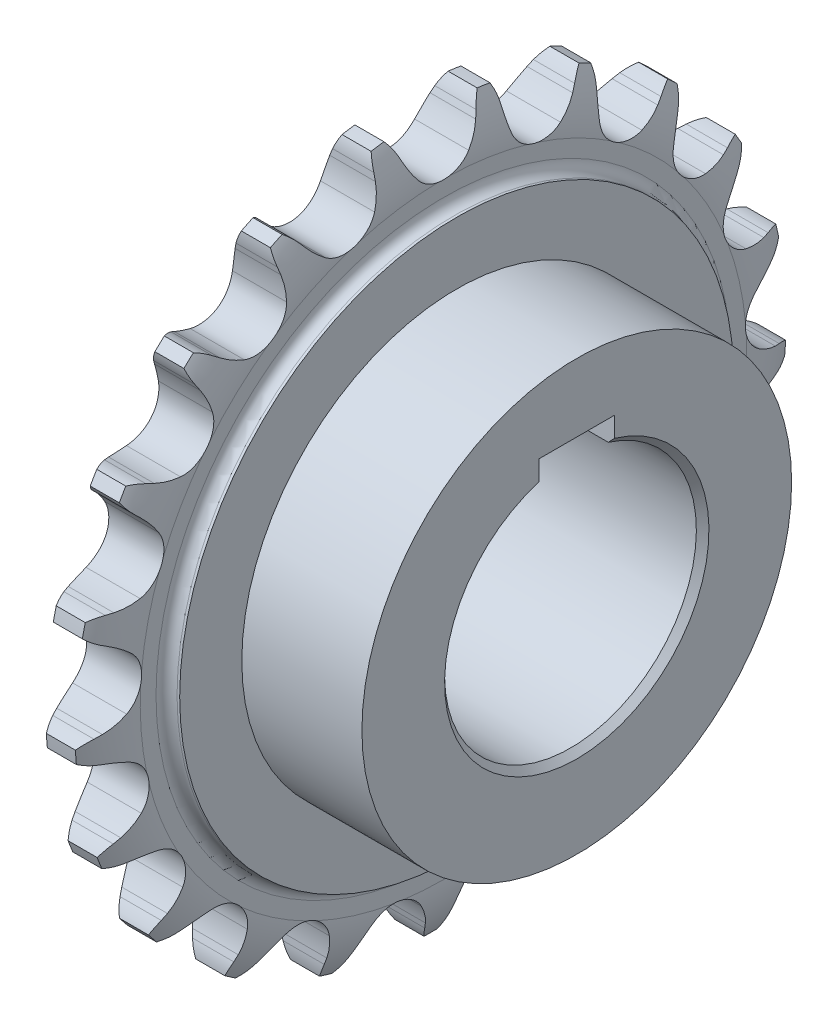
from build123d import *

# Parameters (mm, degrees)
CUT_EXTRUDE_1_DEPTH      = 6.459352492
PATTERN_CIRCULAR_1_COUNT = 21
SKETCH_3_W               = 19.081295016
SKETCH_3_H               = 14.131800766
SKETCH_4_W               = 12
SKETCH_4_H               = 4.221215924
CUT_EXTRUDE_2_DEPTH      = 87.013388292
CHAMFER_1_SIZE           = 1
CHAMFER_3_SIZE           = 1


with BuildPart() as part:
    # 草图1 → 旋转1 (revolve)
    with BuildSketch(Plane.XY, mode=Mode.PRIVATE) as revolve_1_sk:
        with BuildLine():
            Line((-6.459352492, 20), (-6.459352492, 44))
            Line((-6.459352492, 44), (-6.041681994, 44))
            ThreePointArc((-6.041681994, 44), (-4.860331427, 44.489331427), (-4.371, 45.670681994))
            Line((-4.371, 45.670681994), (-4.371, 48.176704985))
            ThreePointArc((-4.371, 48.176704985), (-3.911774122, 52.480340085), (-2.30725, 56.5))
            Line((-2.30725, 56.5), (2.30725, 56.5))
            ThreePointArc((2.30725, 56.5), (3.911774122, 52.480340085), (4.371, 48.176704985))
            Line((4.371, 48.176704985), (4.371, 45.670681994))
            ThreePointArc((4.371, 45.670681994), (4.860331427, 44.489331427), (6.041681994, 44))
            Line((6.041681994, 44), (6.459352492, 44))
            Line((6.459352492, 44), (6.459352492, 20))
            Line((6.459352492, 20), (-6.459352492, 20))
        make_face()
    revolve(revolve_1_sk.sketch.rotate(Axis((-7.9375, 0, 0), (1, 0, 0)), 90), axis=Axis((-7.9375, 0, 0), (1, 0, 0)))

    # 草图2 → 切除-拉伸1 (cut, symmetric)
    with BuildSketch(Plane(origin=(0, 0, 0), x_dir=(0, 0, -1), z_dir=(1, 0, 0))):
        with BuildLine():
            Line((5.852739584, 53.156379816), (6.249341137, 54.112736402))
            ThreePointArc((6.249341137, 54.112736402), (6.752605781, 55.10660921), (7.399855354, 56.013321101))
            ThreePointArc((7.399855354, 56.013321101), (0, 56.5), (-7.399855354, 56.013321101))
            ThreePointArc((-7.399855354, 56.013321101), (-6.752605781, 55.10660921), (-6.249341137, 54.112736402))
            Line((-6.249341137, 54.112736402), (-5.852739584, 53.156379816))
            ThreePointArc((-5.852739584, 53.156379816), (-5.064210074, 51.564909521), (-4.070411778, 50.09286284))
            ThreePointArc((-4.070411778, 50.09286284), (0, 48.101304985), (4.070411778, 50.09286284))
            ThreePointArc((4.070411778, 50.09286284), (5.064210074, 51.564909521), (5.852739584, 53.156379816))
        make_face()
    cut_extrude_1 = extrude(amount=CUT_EXTRUDE_1_DEPTH, both=True, mode=Mode.SUBTRACT)

    # 阵列(圆周)1: 切除-拉伸1 ×21 about axis
    pattern_circular_1_axis = Axis((0, 0, 0), (1, 0, 0))
    for i in range(1, PATTERN_CIRCULAR_1_COUNT):
        add(cut_extrude_1.rotate(pattern_circular_1_axis, i * 360 / PATTERN_CIRCULAR_1_COUNT), mode=Mode.SUBTRACT)

    # 草图3 → 旋转2 (revolve)
    with BuildSketch(Plane.XY, mode=Mode.PRIVATE) as revolve_2_sk:
        with Locations((16, 27.065900383)):
            Rectangle(SKETCH_3_W, SKETCH_3_H)
    revolve(revolve_2_sk.sketch.rotate(Axis((0, 0, 0), (1, 0, 0)), 90), axis=Axis((0, 0, 0), (1, 0, 0)))

    # 草图4 → 切除-拉伸2 (cut, through all)
    with BuildSketch(Plane.ZY.offset(6.459352492)):
        with Locations((0, 21.18939199)):
            Rectangle(SKETCH_4_W, SKETCH_4_H)
    extrude(amount=-CUT_EXTRUDE_2_DEPTH, mode=Mode.SUBTRACT)

    # 倒角1
    chamfer_1_edges = [part.edges().sort_by_distance(p)[0] for p in [
        (-6.459352492, -20, 0),
    ]]
    chamfer(chamfer_1_edges, length=CHAMFER_1_SIZE)

    # 倒角3
    chamfer_3_edges = [part.edges().sort_by_distance(p)[0] for p in [
        (25.540647508, -20, 0),
    ]]
    chamfer(chamfer_3_edges, length=CHAMFER_3_SIZE)


solid = part.part
